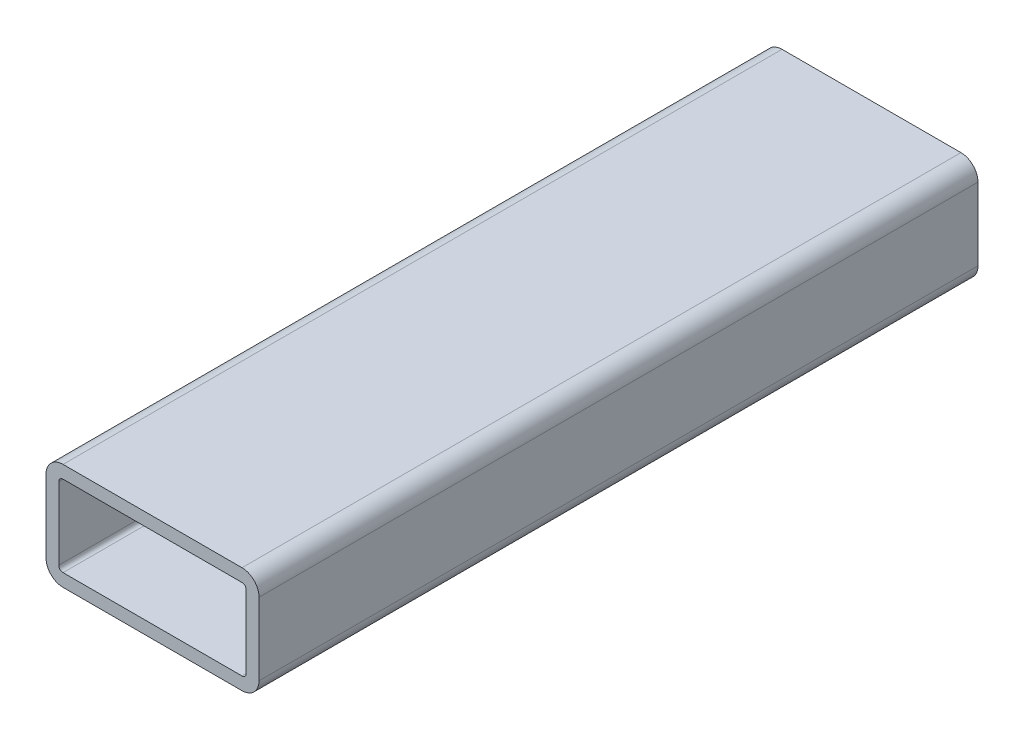
SolidWorks part; units mm, degrees
material "1023 Carbon Steel Plate (SS)"
ref_plane "Front Plane" through (0, 0, 0) normal (0, 0, 1) x (1, 0, 0)
ref_plane "Top Plane" through (0, 0, 0) normal (0, 1, 0) x (1, 0, 0)
ref_plane "Right Plane" through (0, 0, 0) normal (1, 0, 0) x (0, 0, -1)
sketch "Sketch2" plane through (0, 0, 0) normal (0, 0, 1) x (1, 0, 0)
  line L1 (42, 25) -> (-42, 25)
  line L2 (50, 17) -> (50, -17)
  line L3 (42, -25) -> (-42, -25)
  line L4 (-50, 17) -> (-50, -17)
  line L5 (50, 25) -> (-50, -25) construction
  line L6 (50, -25) -> (-50, 25) construction
  arc A0 (-42, -25) -> (-50, -17) centre (-42, -17) cw
  arc A1 (50, -17) -> (42, -25) centre (42, -17) cw
  arc A2 (42, 25) -> (50, 17) centre (42, 17) cw
  arc A3 (-42, 25) -> (-50, 17) centre (-42, 17) ccw
  point P0 (0, 0)
  dimension "D3" = 8
  dimension "D1" = 100
  dimension "D2" = 50
extrude "Boss-Extrude2" add sketch "Sketch2" along normal blind 337.5 contours L4 A0 L3 A1 L2 A2 L1 A3
shell "Shell1" thickness 6
